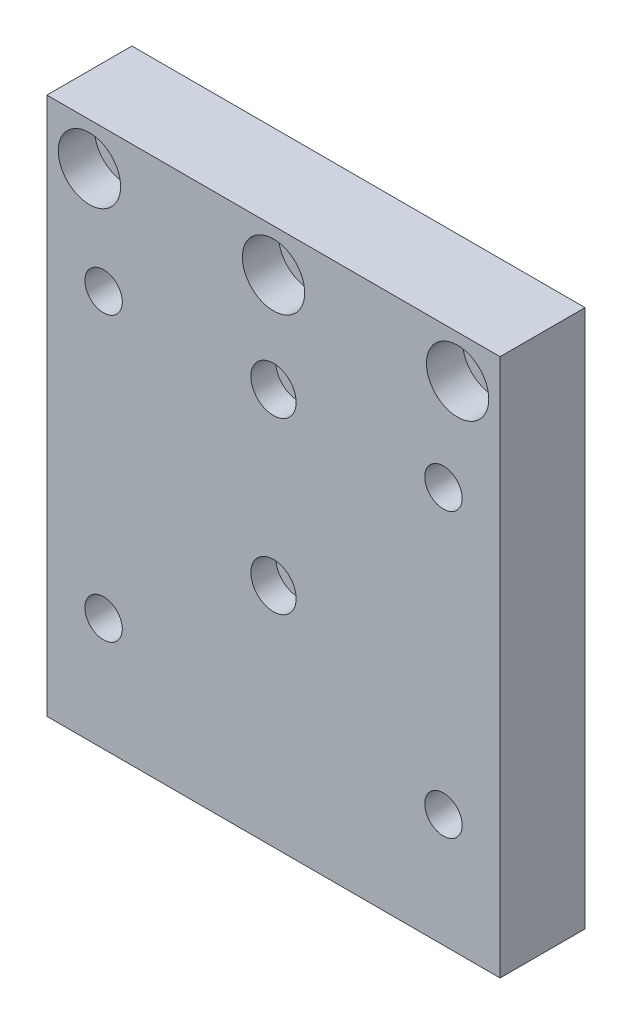
SolidWorks part; units mm, degrees
ref_plane "前视基准面" through (0, 0, 0) normal (0, 0, 1) x (1, 0, 0)
ref_plane "上视基准面" through (0, 0, 0) normal (0, 1, 0) x (1, 0, 0)
ref_plane "右视基准面" through (0, 0, 0) normal (1, 0, 0) x (0, 0, -1)
sketch "草图1" plane through (0, 0, 0) normal (0, 0, 1) x (1, 0, 0)
  line L1 (-40, 47.5) -> (40, 47.5)
  line L2 (-40, 47.5) -> (-40, -47.5)
  line L3 (-40, -47.5) -> (40, -47.5)
  line L4 (40, 47.5) -> (40, -47.5)
  line L5 (-40, 47.5) -> (40, -47.5) construction
  line L6 (-40, -47.5) -> (40, 47.5) construction
  point P0 (0, 0)
  dimension "D1" = 80
  dimension "D2" = 95
extrude "凸台-拉伸1" add sketch "草图1" along normal blind 15
hole_wizard "M4 六角凹头螺钉的柱形沉头孔1" positions "草图2" profile "草图3" counterbore size "M4" standard "ISO" end condition through all
sketch "草图2" plane through (0, 0, 15) normal (0, 0, 1) x (1, 0, 0)
  line L0 (0, 47.5) -> (0, -47.5) construction
  line L1 (40, 47.5) -> (-40, 47.5) construction
  line L2 (-40, -47.5) -> (40, -47.5) construction
  point P0 (0, 22.5)
  point P2 (0, -7.5)
  dimension "D1" = 25
  dimension "D2" = 30
sketch "草图3" plane through (0, 22.5, 15) normal (1, 0, 0) x (0, -1, 0)
  line L0 (0, 0) -> (0, 15)
  line L1 (0, 15) -> (2.25, 15)
  line L3 (2.25, 15) -> (2.25, 4.4)
  line L4 (2.25, 4.4) -> (4, 4.4)
  line L5 (4, 4.4) -> (4, 0)
  line L7 (4, 0) -> (0, 0)
  line L11 (0, -6.35) -> (0, 107.95) construction
  dimension "通孔孔直径" = 4.5
  dimension "通孔孔深度" = 15
  dimension "柱形沉头孔直径" = 8
  dimension "柱形沉头孔深度" = 4.4
hole_wizard "M6 六角凹头螺钉的柱形沉头孔1" positions "草图4" profile "草图5" counterbore size "M6" standard "ISO" end condition through all
sketch "草图4" plane through (0, 0, 0) normal (0, 0, -1) x (-1, 0, 0)
  line L0 (0, 47.5) -> (0, -47.5) construction
  line L1 (-40, 47.5) -> (40, 47.5) construction
  line L2 (40, -47.5) -> (-40, -47.5) construction
  point P0 (-30, 22.5)
  point P2 (30, 22.5)
  point P4 (30, -27.5)
  point P6 (-30, -27.5)
  dimension "D1" = 60
  dimension "D2" = 50
  dimension "D3" = 20
sketch "草图5" plane through (30, 22.5, 0) normal (1, 0, 0) x (0, 1, 0)
  line L0 (0, 0) -> (0, 15)
  line L1 (0, 15) -> (3.3, 15)
  line L3 (3.3, 15) -> (3.3, 6.4)
  line L4 (3.3, 6.4) -> (5.5, 6.4)
  line L5 (5.5, 6.4) -> (5.5, 0)
  line L7 (5.5, 0) -> (0, 0)
  line L11 (0, -6.35) -> (0, 107.95) construction
  dimension "通孔孔直径" = 6.6
  dimension "通孔孔深度" = 15
  dimension "柱形沉头孔直径" = 11
  dimension "柱形沉头孔深度" = 6.4
hole_wizard "M6 六角凹头螺钉的柱形沉头孔2" positions "草图7" profile "草图8" counterbore size "M6" standard "ISO" end condition through all
sketch "草图7" plane through (0, 0, 15) normal (0, 0, 1) x (1, 0, 0)
  line L0 (0, 47.5) -> (0, 0) construction
  line L1 (40, 47.5) -> (-40, 47.5) construction
  point P0 (-32.5, 40)
  point P2 (0, 40)
  point P4 (32.5, 40)
  dimension "D1" = 65
  dimension "D2" = 7.5
sketch "草图8" plane through (-32.5, 40, 15) normal (1, 0, 0) x (0, -1, 0)
  line L0 (0, 0) -> (0, 15)
  line L1 (0, 15) -> (3.3, 15)
  line L3 (3.3, 15) -> (3.3, 6.4)
  line L4 (3.3, 6.4) -> (5.5, 6.4)
  line L5 (5.5, 6.4) -> (5.5, 0)
  line L7 (5.5, 0) -> (0, 0)
  line L11 (0, -6.35) -> (0, 107.95) construction
  dimension "通孔孔直径" = 6.6
  dimension "通孔孔深度" = 15
  dimension "柱形沉头孔直径" = 11
  dimension "柱形沉头孔深度" = 6.4
